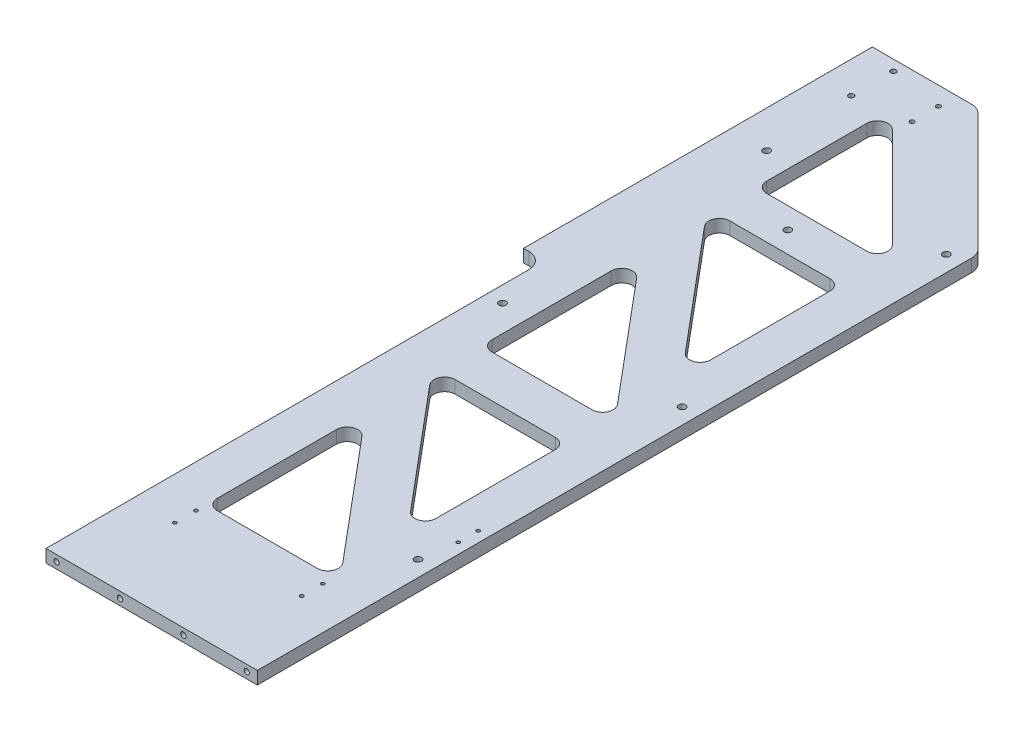
from build123d import *

# Parameters (mm, degrees)
SKETCH_1_W             = 220
SKETCH_1_H             = 330
EXTRUDE_1_DEPTH        = 6
SKETCH_2_W             = 200
SKETCH_2_H             = 472
EXTRUDE_2_DEPTH        = 12
CHAMFER_1_SIZE         = 120
FILLET_2_R             = 15
CUT_EXTRUDE_3_DEPTH    = 12
HOLE_WIZARD_M6_1_D     = 5
HOLE_WIZARD_M6_1_DEPTH = 17
HOLE_WIZARD_M6_1_TIP   = 1.502151548
HOLE_WIZARD_M6_2_D     = 5
HOLE_WIZARD_M6_2_DEPTH = 17
HOLE_WIZARD_M6_2_TIP   = 1.502151548
HOLE_WIZARD_M6_1_2_D   = 6.6
HOLE_WIZARD_M6_2_2_D   = 6.6
HOLE_WIZARD_M6_3_D     = 5
HOLE_WIZARD_M5_1_D     = 4.2
HOLE_WIZARD_M4_1_D     = 3.3
HOLE_WIZARD_M4_2_D     = 3.3


with BuildPart() as part:
    # 草图1 → 凸台-拉伸1 (new, symmetric)
    with BuildSketch(Plane(origin=(0, 0, 0), x_dir=(1, 0, 0), z_dir=(0, 1, 0))):
        Rectangle(SKETCH_1_W, SKETCH_1_H)
    extrude(amount=EXTRUDE_1_DEPTH, both=True)

    # 草图2 → 凸台-拉伸2 (add)
    with BuildSketch(Plane(origin=(0, 6, 0), x_dir=(1, 0, 0), z_dir=(0, 1, 0))):
        with Locations((10, -401)):
            Rectangle(SKETCH_2_W, SKETCH_2_H)
    extrude(amount=-EXTRUDE_2_DEPTH)

    # 倒角1
    chamfer_1_edges = [part.edges().sort_by_distance(p)[0] for p in [
        (110, 0, -165),
    ]]
    chamfer(chamfer_1_edges, length=CHAMFER_1_SIZE)

    # 圆角2
    fillet_2_edges = [part.edges().sort_by_distance(p)[0] for p in [
        (-10, 0, -165),
        (110, 0, -45),
        (-90, 0, 165),
    ]]
    fillet(fillet_2_edges, radius=FILLET_2_R)

    # 草图7 → 切除-拉伸3 (cut)
    with BuildSketch(Plane(origin=(0, 6, 0), x_dir=(1, 0, 0), z_dir=(0, 1, 0))):
        with BuildLine():
            Line((-34.747744438, -45), (60, -45))
            ThreePointArc((60, -45), (67.071067812, -47.928932188), (70, -55))
            Line((70, -55), (70, -167.915964824))
            ThreePointArc((70, -167.915964824), (63.420201433, -177.312891032), (52.339555569, -174.343840921))
            Line((52.339555569, -174.343840921), (-42.408188869, -61.427876097))
            ThreePointArc((-42.408188869, -61.427876097), (-43.810822308, -50.773817383), (-34.747744438, -45))
        make_face()
        with BuildLine():
            Line((-32.339555569, -135.656159079), (62.408188869, -248.572123903))
            ThreePointArc((62.408188869, -248.572123903), (63.810822308, -259.226182617), (54.747744438, -265))
            Line((54.747744438, -265), (-40, -265))
            ThreePointArc((-40, -265), (-47.071067812, -262.071067812), (-50, -255))
            Line((-50, -255), (-50, -142.084035176))
            ThreePointArc((-50, -142.084035176), (-43.420201433, -132.687108968), (-32.339555569, -135.656159079))
        make_face()
        with BuildLine():
            Line((-34.747744438, -305), (60, -305))
            ThreePointArc((60, -305), (67.071067812, -307.928932188), (70, -315))
            Line((70, -315), (70, -427.915964824))
            ThreePointArc((70, -427.915964824), (63.420201433, -437.312891032), (52.339555569, -434.343840921))
            Line((52.339555569, -434.343840921), (-42.408188869, -321.427876097))
            ThreePointArc((-42.408188869, -321.427876097), (-43.810822308, -310.773817383), (-34.747744438, -305))
        make_face()
        with BuildLine():
            Line((-32.339555569, -395.656159079), (62.408188869, -508.572123903))
            ThreePointArc((62.408188869, -508.572123903), (63.810822308, -519.226182617), (54.747744438, -525))
            Line((54.747744438, -525), (-40, -525))
            ThreePointArc((-40, -525), (-47.071067812, -522.071067812), (-50, -515))
            Line((-50, -515), (-50, -402.084035176))
            ThreePointArc((-50, -402.084035176), (-43.420201433, -392.687108968), (-32.339555569, -395.656159079))
        make_face()
        with BuildLine():
            Line((-50, 99.747744438), (-50, 5))
            ThreePointArc((-50, 5), (-47.071067812, -2.071067812), (-40, -5))
            Line((-40, -5), (54.747744438, -5))
            ThreePointArc((54.747744438, -5), (63.986539763, 1.173165676), (61.81881225, 12.071067812))
            Line((61.81881225, 12.071067812), (-32.928932188, 106.81881225))
            ThreePointArc((-32.928932188, 106.81881225), (-43.826834324, 108.986539763), (-50, 99.747744438))
        make_face()
    extrude(amount=-CUT_EXTRUDE_3_DEPTH, mode=Mode.SUBTRACT)

    # Hole Wizard M6 _1
    with Locations(Plane.XY.offset(637)):
        with Locations((-80, 0), (-20, 0), (40, 0), (100, 0)):
            Hole(HOLE_WIZARD_M6_1_D / 2, depth=HOLE_WIZARD_M6_1_DEPTH)
            with Locations((0, 0, -(HOLE_WIZARD_M6_1_DEPTH + HOLE_WIZARD_M6_1_TIP / 2))):  # 118° drill point
                Cone(0, HOLE_WIZARD_M6_1_D / 2, HOLE_WIZARD_M6_1_TIP, mode=Mode.SUBTRACT)

    # Hole Wizard M6 _2
    with Locations(Plane.ZY.offset(110)):
        with Locations((-150, 0), (-90, 0), (-30, 0), (30, 0), (90, 0), (150, 0)):
            Hole(HOLE_WIZARD_M6_2_D / 2, depth=HOLE_WIZARD_M6_2_DEPTH)
            with Locations((0, 0, -(HOLE_WIZARD_M6_2_DEPTH + HOLE_WIZARD_M6_2_TIP / 2))):  # 118° drill point
                Cone(0, HOLE_WIZARD_M6_2_D / 2, HOLE_WIZARD_M6_2_TIP, mode=Mode.SUBTRACT)

    # Hole Wizard M6 _1 2 (through all)
    with Locations(Plane(origin=(0, 6, 0), x_dir=(1, 0, 0), z_dir=(0, 1, 0))):
        with Locations((95, 30), (-75, 30), (-75, -220), (95, -220), (95, -470)):
            Hole(HOLE_WIZARD_M6_1_2_D / 2)

    # Hole Wizard M6 _2 2 (through all)
    with Locations(Plane(origin=(0, 6, 0), x_dir=(1, 0, 0), z_dir=(0, 1, 0))):
        with Locations((0, -25)):
            Hole(HOLE_WIZARD_M6_2_2_D / 2)

    # M6 螺纹孔3 (through all)
    with Locations(Plane(origin=(0, 6, 0), x_dir=(1, 0, 0), z_dir=(0, 1, 0))):
        with Locations((-80, 155), (-80, 115)):
            Hole(HOLE_WIZARD_M6_3_D / 2)

    # M5 螺纹孔1 (through all)
    with Locations(Plane(origin=(0, 6, 0), x_dir=(1, 0, 0), z_dir=(0, 1, 0))):
        with Locations((-30, 147.5), (-30, 122.5)):
            Hole(HOLE_WIZARD_M5_1_D / 2)

    # M4 螺纹孔1 (through all)
    with Locations(Plane(origin=(0, 6, 0), x_dir=(1, 0, 0), z_dir=(0, 1, 0))):
        with Locations((100, -418), (100, -437)):
            Hole(HOLE_WIZARD_M4_1_D / 2)

    # M4 螺纹孔2 (through all)
    with Locations(Plane(origin=(0, -6, 0), x_dir=(-1, 0, 0), z_dir=(0, -1, 0))):
        with Locations((-70, -535), (50, -555), (-70, -555), (50, -535)):
            Hole(HOLE_WIZARD_M4_2_D / 2)


solid = part.part
